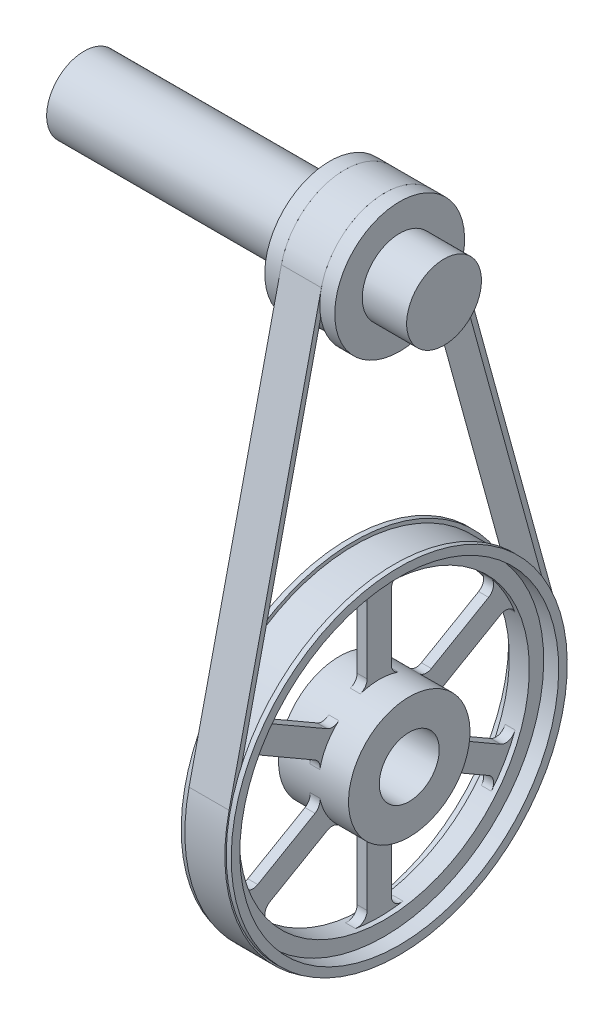
SolidWorks part; units mm, degrees
ref_plane "Front Plane" through (0, 0, 0) normal (0, 0, 1) x (1, 0, 0)
ref_plane "Top Plane" through (0, 0, 0) normal (0, 1, 0) x (1, 0, 0)
ref_plane "Right Plane" through (0, 0, 0) normal (1, 0, 0) x (0, 0, -1)
other "Configuration Table"
sketch "Sketch2" plane through (54.9996, 0, 0) normal (-1, 0, 0) x (0, 0, 1)
  circle A0 centre (-0.9579, -42.4595) radius 3
  circle A1 centre (-0.9579, -42.4595) radius 6.0748
extrude "Boss-Extrude1" add sketch "Sketch2" against normal blind 7
ref_plane "Plane1" through (58.4996, 0, 0) normal (-1, 0, 0) x (0, 0, 1)
sketch "Sketch3" plane through (58.4996, 0, 0) normal (-1, 0, 0) x (0, 0, 1)
  circle A0 centre (-0.9579, -42.4595) radius 15.9473
  circle A1 centre (-0.9579, -42.4595) radius 16.8064
extrude "Boss-Extrude2" add sketch "Sketch3" along normal mid plane 5 separate body
sketch "Sketch4" plane through (58.4996, 0, 0) normal (-1, 0, 0) x (0, 0, 1)
  circle A0 centre (-0.9579, -42.4595) radius 15.9473
  circle A1 centre (-0.9579, -42.4595) radius 14.512
extrude "Boss-Extrude3" add sketch "Sketch4" along normal mid plane 2
sketch "Sketch5" plane through (58.4996, 0, 0) normal (-1, 0, 0) x (0, 0, 1)
  line L0 (10.9592, -34.1781) -> (3.5904, -38.4325)
  line L2 (-2.1712, -27.9983) -> (-2.1712, -36.5071)
  line L4 (0.2554, -27.9983) -> (0.2554, -36.5071)
  line L5 (-1.9008, -27.9781) -> (-0.0565, -36.4519) construction
  line L6 (12.1725, -36.2796) -> (4.8037, -40.534)
  line L7 (11.1119, -34.4022) -> (4.6955, -40.2363) construction
  line L8 (12.1725, -48.6394) -> (4.8037, -44.385)
  line L9 (10.9592, -50.7408) -> (3.5904, -46.4864)
  line L10 (12.0548, -48.8836) -> (3.7941, -46.2439) construction
  line L11 (0.2554, -56.9207) -> (0.2554, -48.4119)
  line L12 (-2.1712, -56.9207) -> (-2.1712, -48.4119)
  line L13 (-0.015, -56.9408) -> (-1.8593, -48.4671) construction
  line L14 (-12.875, -50.7408) -> (-5.5062, -46.4864)
  line L15 (-14.0883, -48.6394) -> (-6.7195, -44.385)
  line L16 (-13.0277, -50.5168) -> (-6.6113, -44.6827) construction
  line L17 (-14.0883, -36.2796) -> (-6.7195, -40.534)
  line L18 (-12.875, -34.1781) -> (-5.5062, -38.4325)
  line L19 (-13.9706, -36.0354) -> (-5.7099, -38.6751) construction
  circle A0 centre (-0.9579, -42.4595) radius 14.512 construction
  arc A1 (0.2554, -27.9983) -> (-2.1712, -27.9983) centre (-0.9579, -42.4595) ccw
  arc A2 (12.1725, -36.2796) -> (10.9592, -34.1781) centre (-0.9579, -42.4595) ccw
  circle A3 centre (-0.9579, -42.4595) radius 6.0748
  arc A4 (0.2554, -36.5071) -> (-2.1712, -36.5071) centre (-0.9579, -42.4595) ccw
  arc A5 (4.8037, -40.534) -> (3.5904, -38.4325) centre (-0.9579, -42.4595) ccw
  arc A6 (10.9592, -50.7408) -> (12.1725, -48.6394) centre (-0.9579, -42.4595) ccw
  arc A7 (3.5904, -46.4864) -> (4.8037, -44.385) centre (-0.9579, -42.4595) ccw
  arc A8 (-2.1712, -56.9207) -> (0.2554, -56.9207) centre (-0.9579, -42.4595) ccw
  arc A9 (-2.1712, -48.4119) -> (0.2554, -48.4119) centre (-0.9579, -42.4595) ccw
  arc A10 (-14.0883, -48.6394) -> (-12.875, -50.7408) centre (-0.9579, -42.4595) ccw
  arc A11 (-6.7195, -44.385) -> (-5.5062, -46.4864) centre (-0.9579, -42.4595) ccw
  arc A12 (-12.875, -34.1781) -> (-14.0883, -36.2796) centre (-0.9579, -42.4595) ccw
  arc A13 (-5.5062, -38.4325) -> (-6.7195, -40.534) centre (-0.9579, -42.4595) ccw
  point P0 (-0.9579, -32.3105)
  point P12 (7.8314, -37.385)
  point P21 (7.8314, -47.534)
  point P28 (-0.9579, -52.6085)
  point P35 (-9.7472, -47.534)
  point P42 (-9.7472, -37.385)
  point P49 (-0.9579, -42.4595)
  dimension "D1" = 0
  dimension "D2" = 6
extrude "Boss-Extrude4" add sketch "Sketch5" along normal mid plane 1
fillet "Fillet1" radius 1 4 edges at (58.4996, -40.534, -6.7195) (58.4996, -36.2796, -14.0883) (58.4996, -38.4325, -5.5062) (58.4996, -34.1781, -12.875)
fillet "Fillet2" radius 1 20 edges at (58.4996, -46.4864, -5.5062) (58.4996, -44.385, -6.7195) (58.4996, -48.6394, -14.0883) (58.4996, -50.7408, -12.875) (58.4996, -56.9207, -2.1712) (58.4996, -48.4119, -2.1712) (58.4996, -56.9207, 0.2554) (58.4996, -48.4119, 0.2554) (58.4996, -50.7408, 10.9592) (58.4996, -46.4864, 3.5904) (58.4996, -44.385, 4.8037) (58.4996, -48.6394, 12.1725) (58.4996, -36.2796, 12.1725) (58.4996, -40.534, 4.8037) (58.4996, -38.4325, 3.5904) (58.4996, -34.1781, 10.9592) (58.4996, -27.9983, 0.2554) (58.4996, -36.5071, 0.2554) (58.4996, -36.5071, -2.1712) (58.4996, -27.9983, -2.1712)
sketch "Sketch6" plane through (58.4996, 0, 0) normal (-1, 0, 0) x (0, 0, 1)
  circle A0 centre (-0.9579, -42.4595) radius 16.4422
  circle A1 centre (-0.9579, -42.4595) radius 19.0884
extrude "Cut-Extrude1" cut sketch "Sketch6" against normal mid plane 4
sketch "Sketch7" plane through (34.4372, 0, 0) normal (1, 0, 0) x (0, 0, -1)
  circle A0 centre (0, 0.4922) radius 3.7422
extrude "Boss-Extrude5" add sketch "Sketch7" along normal blind 32 and the other way blind 4 separate body
sketch "Sketch8" plane through (54.9996, 0, 0) normal (-1, 0, 0) x (0, 0, 1)
  circle A0 centre (0, 0.4922) radius 6.4919
  circle A2 centre (0, 0.4922) radius 3.7422
  circle A3 centre (0, 0.4922) radius 3.7422
  dimension "D1" = 0
extrude "Boss-Extrude6" add sketch "Sketch8" against normal up to surface (7 mm away) up to face at (61.9996, -45.4595, -0.9579)
sketch "Sketch9" plane through (58.4996, 0, 0) normal (-1, 0, 0) x (0, 0, 1)
  circle A0 centre (0, 0.4922) radius 5.9978
  circle A1 centre (0, 0.4922) radius 7.1734
extrude "Cut-Extrude2" cut sketch "Sketch9" against normal mid plane 4
sketch "Sketch11" plane through (60.4996, 0, 0) normal (-1, 0, 0) x (0, 0, 1)
  line L0 (-6.2602, 2.2113) -> (-17.2953, -37.9731)
  line L1 (-5.7839, 2.0797) -> (-16.8137, -38.1077)
  line L2 (0, 0.4922) -> (-0.9579, -42.4595) construction
  line L3 (5.849, 1.8202) -> (15.0762, -38.8189)
  line L4 (6.3306, 1.9305) -> (15.5632, -38.7059)
  circle A0 centre (0, 0.4922) radius 5.9978 construction
  arc A3 (5.849, 1.8202) -> (-5.7839, 2.0797) centre (0, 0.4922) ccw
  circle A4 centre (-0.9579, -42.4595) radius 16.4422 construction
  arc A7 (-16.8137, -38.1077) -> (15.0762, -38.8189) centre (-0.9579, -42.4595) ccw
  arc A8 (-17.2953, -37.9731) -> (15.5632, -38.7059) centre (-0.9579, -42.4595) ccw
  arc A9 (6.3306, 1.9305) -> (-6.2602, 2.2113) centre (0, 0.4922) ccw
extrude "Boss-Extrude7" add sketch "Sketch11" along normal up to surface (4 mm away) separate body up to face at (56.4996, -5.9997, 0)
